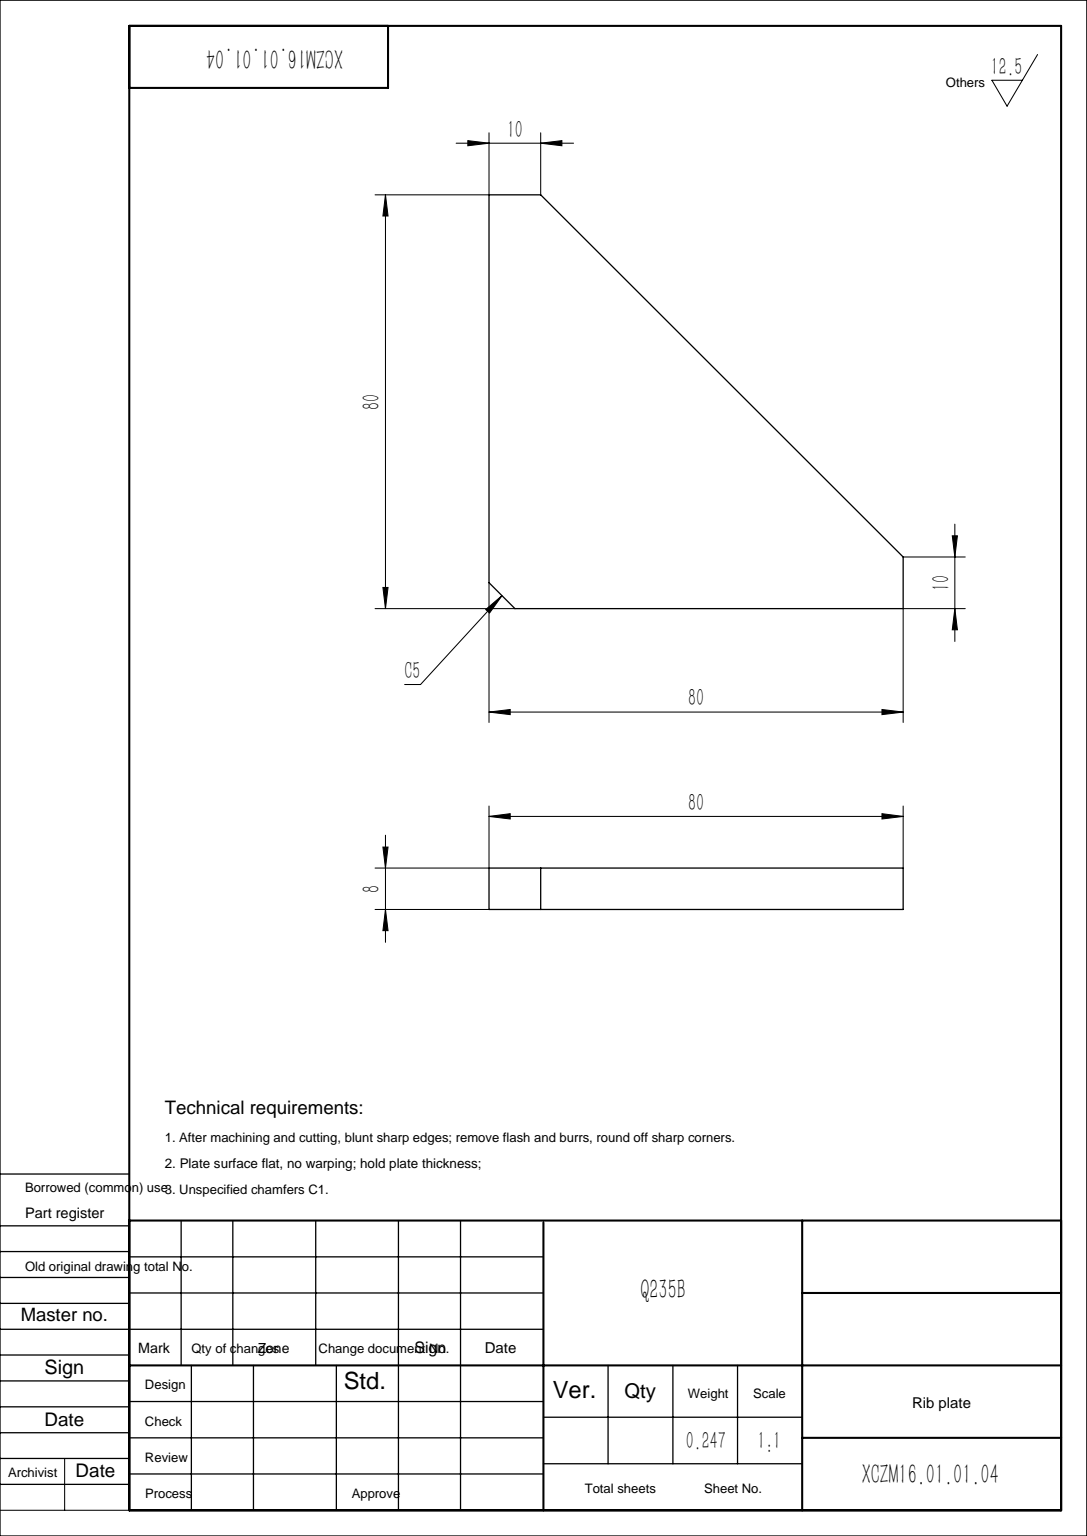
SolidWorks part; units mm, degrees
material "Q235B"
ref_plane "Front Plane" through (0, 0, 0) normal (0, 0, 1) x (1, 0, 0)
ref_plane "Top Plane" through (0, 0, 0) normal (0, 1, 0) x (1, 0, 0)
ref_plane "Right Plane" through (0, 0, 0) normal (1, 0, 0) x (0, 0, -1)
sketch "Sketch1" plane through (0, 0, 0) normal (0, 0, 1) x (1, 0, 0)
  line L0 (0, 80) -> (0, 0)
  line L1 (0, 0) -> (80, 0)
  line L2 (80, 0) -> (80, 10)
  line L3 (80, 10) -> (10, 80)
  line L4 (10, 80) -> (0, 80)
  dimension "D1" = 80
  dimension "D2" = 10
extrude "Boss-Extrude1" add sketch "Sketch1" along normal blind 8
chamfer "Chamfer1" distance 5 angle 45 1 edges at (0, 0, 4)
